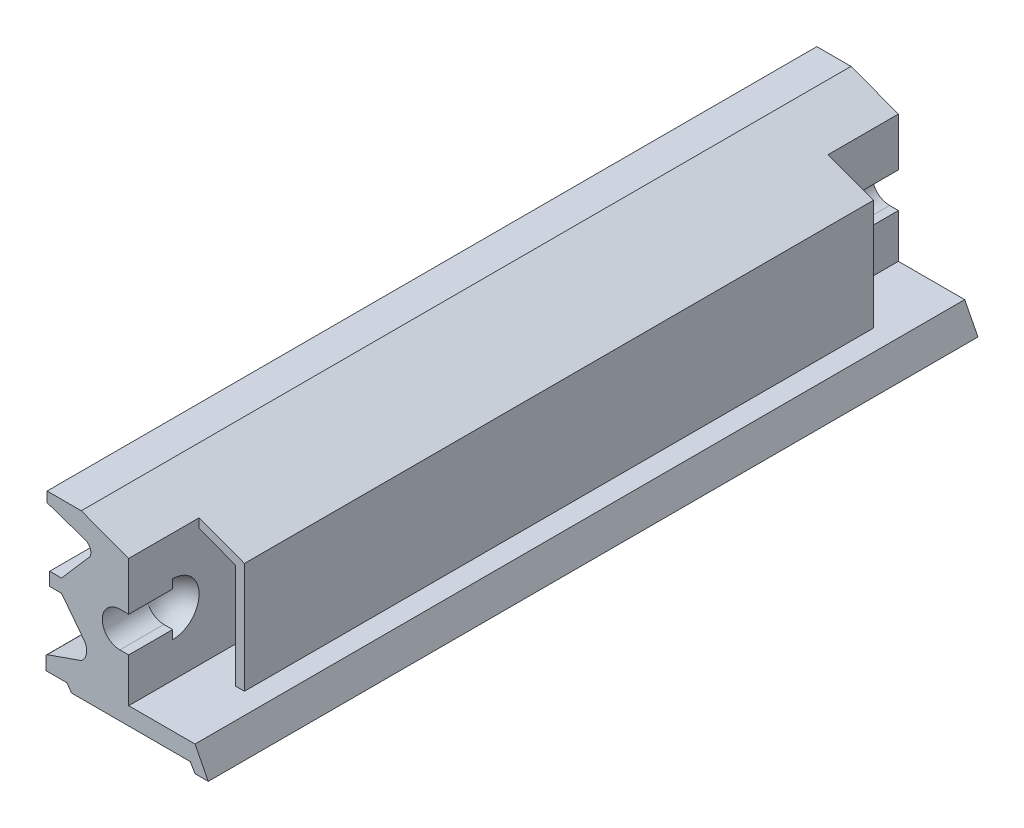
from build123d import *

# Parameters (mm, degrees)
EXTRUDE_1_DEPTH     = 1750
CUT_EXTRUDE_2_DEPTH = 100
CUT_REVOLVE_1_ANGLE = 90
EXTRUDE_2_DEPTH     = 1430


with BuildPart() as part:
    # 草图1 → 凸台-拉伸1 (new body)
    with BuildSketch(Plane.XY):
        with BuildLine():
            Line((-130, -144.49593989), (0, -144.49593989))
            Line((0, -144.49593989), (140, -144.49593989))
            Line((140, -144.49593989), (150.772266034, -162.999521413))
            Line((150.772266034, -162.999521413), (180.947633082, -162.999521413))
            Line((180.947633082, -162.999521413), (150.772266034, -104.49593989))
            Line((150.772266034, -104.49593989), (0, -104.49593989))
            Line((0, -104.49593989), (0, -4.49593989))
            Line((0, -4.49593989), (0, 75.50406011))
            Line((0, 75.50406011), (0, 185.50406011))
            Line((0, 185.50406011), (-107.776879674, 225.507843927))
            Line((-107.776879674, 225.507843927), (-185.49687967, 225.507843927))
            Line((-185.49687967, 225.507843927), (-185.49687967, 202.507843927))
            Line((-185.49687967, 202.507843927), (-99.70724302, 172.98245945))
            add(Edge.make_bspline(
                [(-99.70724302, 172.98245945), (-86.12473236, 169.546572985), (-80.854596401, 148.963344023), (-92.316673431, 140.10859264)],
                knots=[0, 0, 0, 0, 1, 1, 1, 1], degree=3))
            Line((-92.316673431, 140.10859264), (-152.70724302, 70.507843927))
            Line((-152.70724302, 70.507843927), (-179.70724302, 70.507843927))
            Line((-179.70724302, 70.507843927), (-179.70724302, 40.507843927))
            Line((-179.70724302, 40.507843927), (-152.70724302, 40.507843927))
            Line((-152.70724302, 40.507843927), (-102.0083923, -25.203763773))
            ThreePointArc((-102.0083923, -25.203763773), (-95.691769777, -48.530872609), (-107.72, -69.492156073))
            Line((-107.72, -69.492156073), (-185.49687967, -96.73098688))
            add(Edge.make_bspline(
                [(-187.99699364, -99.49593989), (-187.263883629, -97.683704139), (-185.49687967, -96.73098688)],
                knots=[0, 0, 0, 1, 1, 1], degree=2))
            Line((-187.99699364, -99.49593989), (-187.99699364, -129.49593989))
            Line((-187.99699364, -129.49593989), (-140.29956323, -129.49593989))
            Line((-140.29956323, -129.49593989), (-130, -144.49593989))
        make_face()
    extrude(amount=-EXTRUDE_1_DEPTH)

    # 草图2 → 切除-拉伸2 (cut)
    with BuildSketch(Plane.XY):
        with BuildLine():
            Line((0, 75.50406011), (0, -4.49593989))
            Line((0, -4.49593989), (-20, -4.49593989))
            ThreePointArc((-20, -4.49593989), (-60, 35.50406011), (-20, 75.50406011))
            Line((-20, 75.50406011), (0, 75.50406011))
        make_face()
    cut_extrude_2 = extrude(amount=-CUT_EXTRUDE_2_DEPTH, mode=Mode.SUBTRACT)

    # 草图4 → 切除-旋转1 (revolve, cut)
    with BuildSketch(Plane(origin=(0, 0, 0), x_dir=(0, 0, -1), z_dir=(1, 0, 0))):
        with BuildLine():
            Line((100, 95.50406011), (100, -24.49593989))
            ThreePointArc((100, -24.49593989), (160, 35.50406011), (100, 95.50406011))
        make_face()
    cut_revolve_1 = revolve(axis=Axis((0, 95.50406011, -100), (0, 1, 0)), revolution_arc=CUT_REVOLVE_1_ANGLE, mode=Mode.SUBTRACT)

    # 镜向1: 切除-拉伸2, 切除-旋转1 across plane
    add(cut_extrude_2.mirror(Plane.XY.offset(-875)), mode=Mode.SUBTRACT)
    add(cut_revolve_1.mirror(Plane.XY.offset(-875)), mode=Mode.SUBTRACT)

    # 草图6 → 凸台-拉伸2 (add)
    with BuildSketch(Plane.XY.offset(-160)):
        Polygon((0, 185.50406011), (63.207169624, 162.043314569), (103.142950665, 147.220262017), (103.142950665, -104.49593989), (83.175060144, -104.49593989), (83.175060144, 133.726046688), (0, 164.598318505), align=None)
    extrude(amount=-EXTRUDE_2_DEPTH)


solid = part.part
